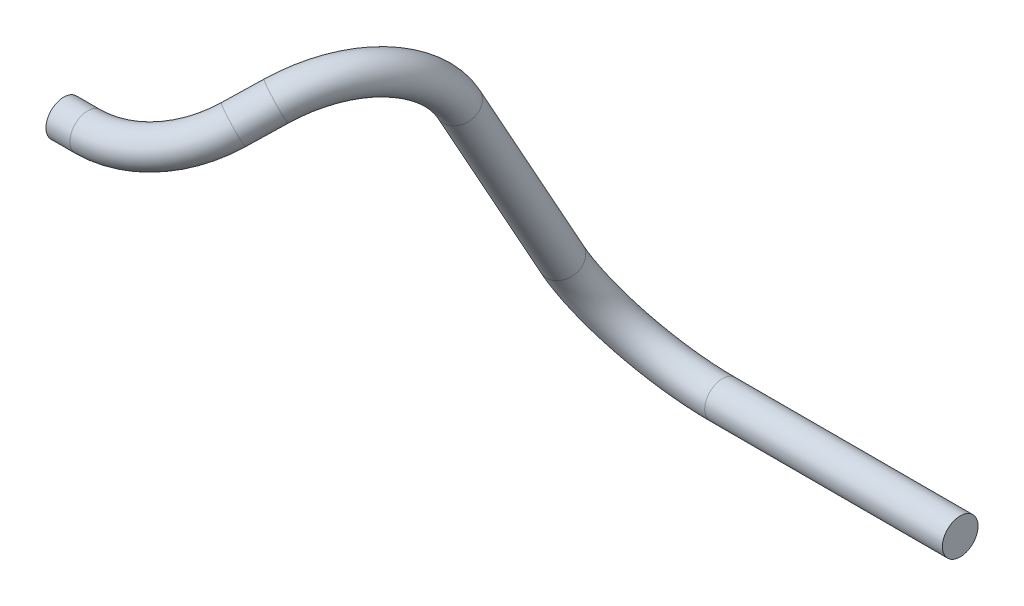
SolidWorks part; units mm, degrees
ref_plane "Front Plane" through (0, 0, 0) normal (0, 0, 1) x (1, 0, 0)
ref_plane "Top Plane" through (0, 0, 0) normal (0, 1, 0) x (1, 0, 0)
ref_plane "Right Plane" through (0, 0, 0) normal (1, 0, 0) x (0, 0, -1)
sketch3d "3DSketch1"
  line L0 (-19.3983, 55.9787, 2.2549) -> (-16.7157, 55.9787, 2.2549)
  line L1 (-6.0476, 59.1236, -3.4396) -> (-4.2699, 60.7921, -6.461)
  line L2 (0.9829, 55.5078, -21.7084) -> (0.4883, 34.1679, -33.7846)
  line L3 (12.4859, 23.5136, -39.8138) -> (39.1717, 23.5136, -39.8138)
  arc A2 (12.4859, 23.5136, -39.8138) -> (0.4883, 34.1679, -33.7846) centre (12.4859, 33.9573, -33.9037) ccw
  arc A3 (0.9829, 55.5078, -21.7084) -> (-4.2699, 60.7921, -6.461) centre (-4.5119, 50.3505, -12.3698) ccw
  arc A4 (-6.0476, 59.1236, -3.4396) -> (-16.7157, 55.9787, 2.2549) centre (-16.7157, 61.7799, -8.2496) ccw
  point P18 (0.2414, 23.5136, -39.8138)
  point P19 (12.4859, 39.8673, -44.3475)
  point P22 (1.2249, 65.9494, -15.7996)
  point P23 (6.1534, 47.4566, -7.6926)
  point P26 (-9.3983, 55.9787, 2.2549)
  point P27 (-16.7157, 51.2754, -14.0509)
  dimension "D2" = 12
  dimension "D1" = 10
  dimension "D3" = 90
ref_plane "Plane1" through (-19.3983, 0, 0) normal (1, 0, 0) x (0, 0, -1)
sketch "Sketch2" plane through (-19.3983, 0, 0) normal (1, 0, 0) x (0, 0, -1)
  circle A0 centre (-2.2549, 55.9787) radius 2
  dimension "D1" = 4
sweep "Sweep1" add profiles "Sketch2" path "3DSketch1"
